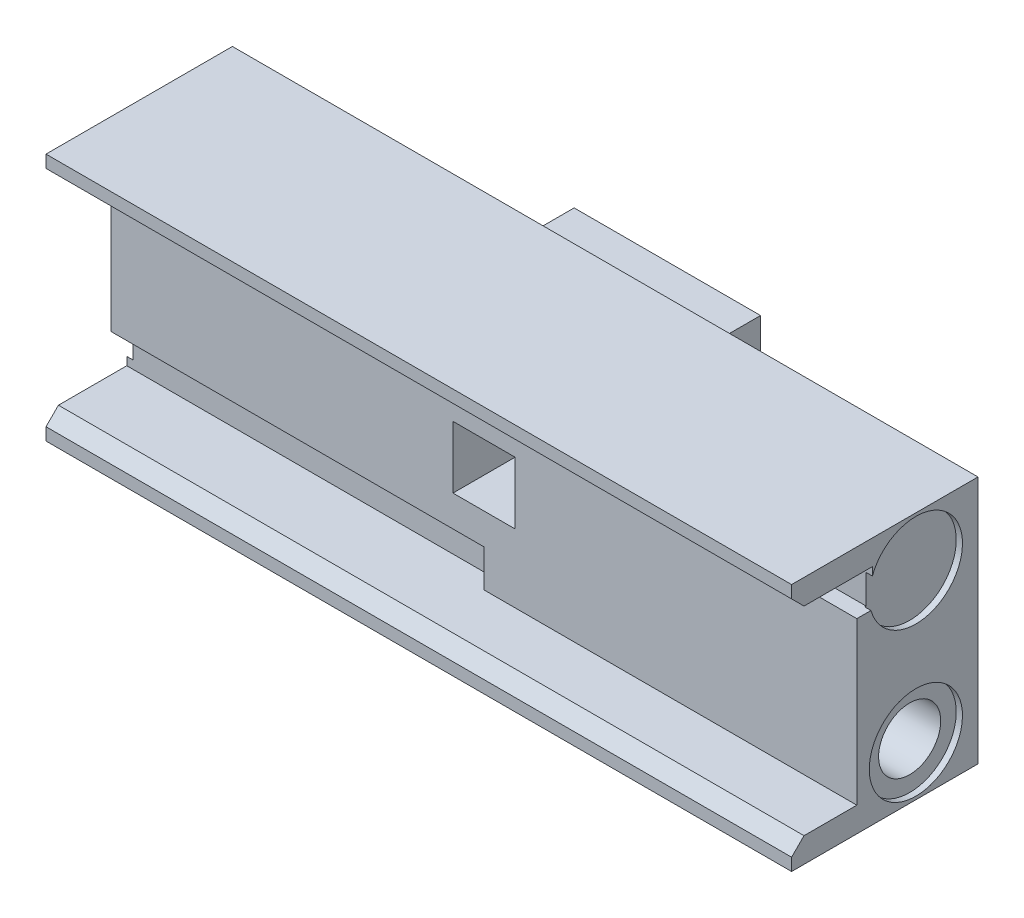
from build123d import *

# Parameters (mm, degrees)
SKETCH1_W           = 120
SKETCH1_H           = 40
BOSS_EXTRUDE1_DEPTH = 30
CUT_EXTRUDE1_DEPTH  = 70
CUT_EXTRUDE2_DEPTH  = 60
SKETCH5_W           = 30
SKETCH5_H           = 30
BOSS_EXTRUDE2_DEPTH = 10
SKETCH7_W           = 10
SKETCH7_H           = 10
CUT_EXTRUDE4_DEPTH  = 10
CHAMFER1_SIZE       = 2
SKETCH6_R           = 7.5
CUT_EXTRUDE5_DEPTH  = 1
SKETCH9_R           = 5
CUT_EXTRUDE6_DEPTH  = 55
SKETCH10_R          = 5
CUT_EXTRUDE7_DEPTH  = 55


with BuildPart() as part:
    # Sketch1 → Boss-Extrude1 (new body)
    with BuildSketch(Plane.XY):
        Rectangle(SKETCH1_W, SKETCH1_H)
    extrude(amount=BOSS_EXTRUDE1_DEPTH)

    # Sketch3 → Cut-Extrude1 (cut)
    with BuildSketch(Plane(origin=(60, 0, 0), x_dir=(0, 0, -1), z_dir=(1, 0, 0))):
        Polygon((-30, 16), (-17, 16), (-17, 10), (-19.5, 10), (-19.5, -16), (-30, -16), align=None)
    extrude(amount=-CUT_EXTRUDE1_DEPTH, mode=Mode.SUBTRACT)

    # Sketch4 → Cut-Extrude2 (cut)
    with BuildSketch(Plane.ZY.offset(60)):
        Polygon((30, 16), (19.5, 16), (19.5, -10), (17, -10), (17, -16), (30, -16), align=None)
    extrude(amount=-CUT_EXTRUDE2_DEPTH, mode=Mode.SUBTRACT)

    # Sketch5 → Boss-Extrude2 (add)
    with BuildSketch(Plane(origin=(0, 0, 0), x_dir=(-1, 0, 0), z_dir=(0, 0, -1))):
        Rectangle(SKETCH5_W, SKETCH5_H)
    extrude(amount=BOSS_EXTRUDE2_DEPTH)

    # Sketch7 → Cut-Extrude4 (cut)
    with BuildSketch(Plane.XY.offset(19.5)):
        Rectangle(SKETCH7_W, SKETCH7_H)
    extrude(amount=-CUT_EXTRUDE4_DEPTH, mode=Mode.SUBTRACT)

    # Chamfer1
    chamfer1_edges = [part.edges().sort_by_distance(p)[0] for p in [
        (0, -16, 30),
        (0, 16, 30),
    ]]
    chamfer(chamfer1_edges, length=CHAMFER1_SIZE)

    # Sketch6 → Cut-Extrude5 (cut)
    with BuildSketch(Plane(origin=(60, 0, 0), x_dir=(0, 0, -1), z_dir=(1, 0, 0))):
        with Locations((-10, 12)):
            Circle(SKETCH6_R)
        with Locations(Location((-10, -12, 0), (0, 0, 90))):
            Circle(SKETCH6_R)
    cut_extrude5 = extrude(amount=-CUT_EXTRUDE5_DEPTH, mode=Mode.SUBTRACT)

    # Sketch9 → Cut-Extrude6 (cut)
    with BuildSketch(Plane(origin=(59, 0, 0), x_dir=(0, 0, -1), z_dir=(1, 0, 0))):
        with Locations(Location((-10, -12, 0), (0, 0, 90))):
            Circle(SKETCH9_R)
    extrude(amount=-CUT_EXTRUDE6_DEPTH, mode=Mode.SUBTRACT)

    # Mirror1: Cut-Extrude5 across plane
    add(cut_extrude5.mirror(Plane(origin=(0, 0, 0), x_dir=(0, 0, 1), z_dir=(1, 0, 0))), mode=Mode.SUBTRACT)

    # Sketch10 → Cut-Extrude7 (cut)
    with BuildSketch(Plane.ZY.offset(59)):
        with Locations(Location((10, 12, 0), (0, 0, 270))):
            Circle(SKETCH10_R)
    extrude(amount=-CUT_EXTRUDE7_DEPTH, mode=Mode.SUBTRACT)


solid = part.part
